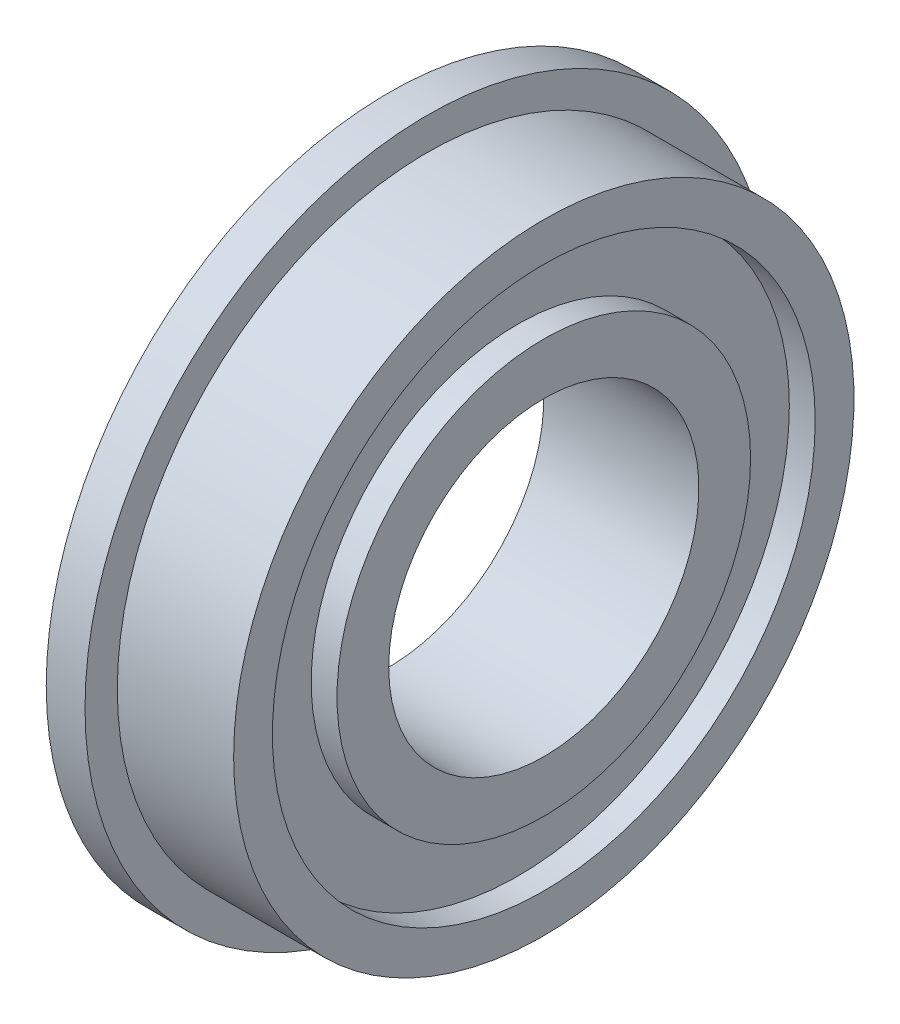
SolidWorks part; units mm, degrees
ref_plane "Front Plane" through (0, 0, 0) normal (0, 0, 1) x (1, 0, 0)
ref_plane "Top Plane" through (0, 0, 0) normal (0, 1, 0) x (1, 0, 0)
ref_plane "Right Plane" through (0, 0, 0) normal (1, 0, 0) x (0, 0, -1)
sketch "Sketch1" plane through (0, 0, 0) normal (0, 0, 1) x (1, 0, 0)
  line L0 (0, 0) -> (6, 0) construction
  line L1 (6, 0) -> (6, 12)
  line L2 (6, 12) -> (1.5, 12)
  line L3 (1.5, 12) -> (1.5, 13.25)
  line L4 (1.5, 13.25) -> (0, 13.25)
  line L5 (0, 13.25) -> (0, 6)
  line L6 (0, 6) -> (6, 6)
  line L7 (0, 6) -> (0, 0)
  dimension "D1" = 12
  dimension "D2" = 24
  dimension "D3" = 6
  dimension "D4" = 1.5
  dimension "D5" = 26.5
revolve "Revolve1" add sketch "Sketch1" angle 360 about L0
sketch "Sketch2" plane through (6, 0, 0) normal (1, 0, 0) x (0, 0, -1)
  circle A0 centre (0, 0) radius 8
  circle A1 centre (0, 0) radius 10.5
  dimension "D1" = 21
  dimension "D2" = 16
extrude "Cut-Extrude1" cut sketch "Sketch2" against normal blind 1
sketch "Sketch3" plane through (0, 0, 0) normal (-1, 0, 0) x (0, 0, 1)
  circle A0 centre (0, 0) radius 8 construction
  circle A1 centre (0, 0) radius 8
  circle A2 centre (0, 0) radius 10.5 construction
  circle A3 centre (0, 0) radius 10.5
extrude "Cut-Extrude2" cut sketch "Sketch3" against normal blind 1
